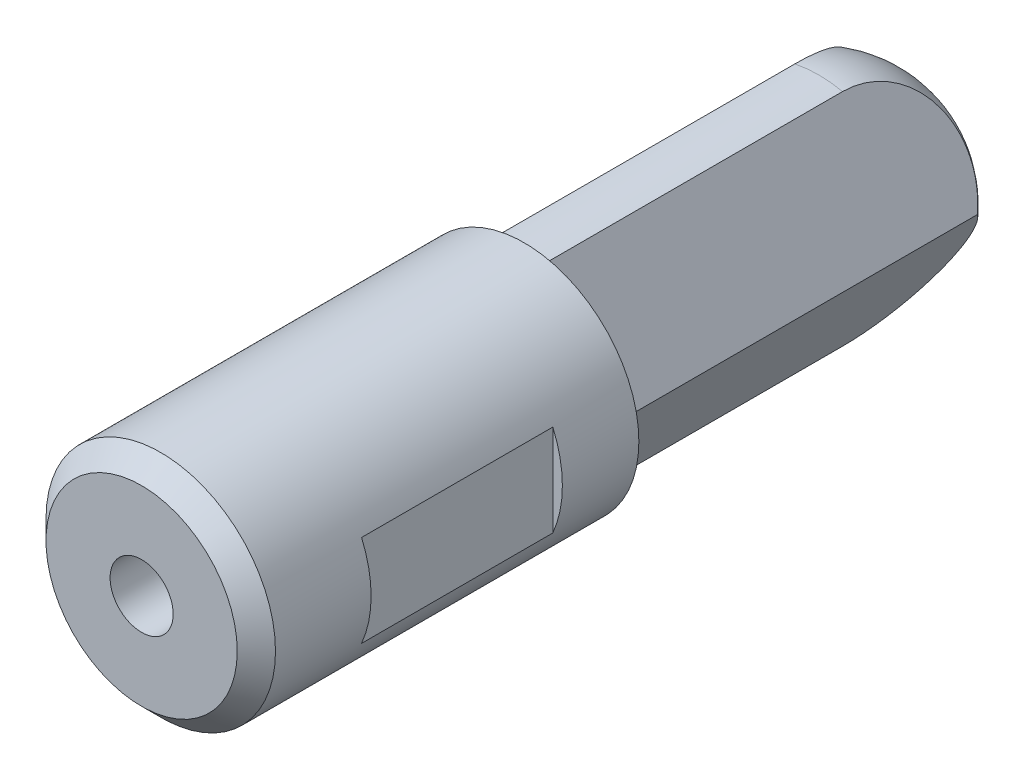
from build123d import *

# Parameters (mm, degrees)
SKETCH1_R               = 5.9
BOSS_EXTRUDE1_DEPTH     = 35.4
M4_TAPPED_HOLE1_D       = 3.3
M4_TAPPED_HOLE1_DEPTH   = 10.1
M4_TAPPED_HOLE1_TIP     = 0.991420021
SKETCH5_R               = 6
SKETCH5_R_2             = 4
BOSS_EXTRUDE2_DEPTH     = 20
CHAMFER1_SIZE           = 1
CUT_EXTRUDE1_DEPTH      = 37.402747149
CUT_EXTRUDE1_DEPTH_BACK = 37.402747149
SKETCH6_W               = 2.026292368
SKETCH6_H               = 10
SKETCH7_OUTSIDE_W       = 22.93
SKETCH7_OUTSIDE_H       = 22.93
CUT_EXTRUDE2_DEPTH      = 23.927930565


with BuildPart() as part:
    # Sketch1 → Boss-Extrude1 (new body)
    with BuildSketch(Plane.XY):
        Circle(SKETCH1_R)
    extrude(amount=BOSS_EXTRUDE1_DEPTH)

    # Sketch2 → Revolve1 (revolve)
    with BuildSketch(Plane(origin=(0, 0, 0), x_dir=(1, 0, 0), z_dir=(0, 1, 0))):
        with BuildLine():
            Line((0, 5.9), (0, 0))
            Line((0, 0), (-5.9, 0))
            ThreePointArc((-5.9, 0), (-4.171930009, 4.171930009), (0, 5.9))
        make_face()
    revolve(axis=Axis((0, 0, -5.9), (0, 0, 1)))

    # M4 Tapped Hole1
    with Locations(Plane.XY.offset(35.4)):
        with Locations((0, 0)):
            Hole(M4_TAPPED_HOLE1_D / 2, depth=M4_TAPPED_HOLE1_DEPTH)
            with Locations((0, 0, -(M4_TAPPED_HOLE1_DEPTH + M4_TAPPED_HOLE1_TIP / 2))):  # 118° drill point
                Cone(0, M4_TAPPED_HOLE1_D / 2, M4_TAPPED_HOLE1_TIP, mode=Mode.SUBTRACT)

    # Sketch5 → Boss-Extrude2 (add)
    with BuildSketch(Plane.XY.offset(35.4)):
        Circle(SKETCH5_R)
        Circle(SKETCH5_R_2, mode=Mode.SUBTRACT)
    extrude(amount=-BOSS_EXTRUDE2_DEPTH)

    # Chamfer1
    chamfer1_edges = [part.edges().sort_by_distance(p)[0] for p in [
        (-6, 0, 35.4),
    ]]
    chamfer(chamfer1_edges, length=CHAMFER1_SIZE)

    # Sketch6 → Cut-Extrude1 (cut, two sides: drawn at the far end of the back side and taken through both)
    with BuildSketch(Plane(origin=(0, 0, 0), x_dir=(1, 0, 0), z_dir=(0, 1, 0)).offset(-CUT_EXTRUDE1_DEPTH_BACK)):
        with Locations((-6.513146184, -24.4)):
            Rectangle(SKETCH6_W, SKETCH6_H)
        with Locations((6.513146184, -24.4)):
            Rectangle(SKETCH6_W, SKETCH6_H)
    extrude(amount=CUT_EXTRUDE1_DEPTH + CUT_EXTRUDE1_DEPTH_BACK, mode=Mode.SUBTRACT)

    # Sketch7 outside → Cut-Extrude2 (cut, through all)
    with BuildSketch(Plane(origin=(0, 0, 15.4), x_dir=(-1, 0, 0), z_dir=(0, 0, -1))):
        Rectangle(SKETCH7_OUTSIDE_W, SKETCH7_OUTSIDE_H)
        with BuildLine():
            Line((-1.25, 5.766064516), (-4.5790389, 0))
            Line((-4.5790389, 0), (-1.25, -5.766064516))
            ThreePointArc((-1.25, -5.766064516), (0, -5.9), (1.25, -5.766064516))
            Line((1.25, -5.766064516), (4.5790389, 0))
            Line((4.5790389, 0), (1.25, 5.766064516))
            ThreePointArc((1.25, 5.766064516), (0, 5.9), (-1.25, 5.766064516))
        make_face(mode=Mode.SUBTRACT)
    extrude(amount=CUT_EXTRUDE2_DEPTH, mode=Mode.SUBTRACT)


solid = part.part
